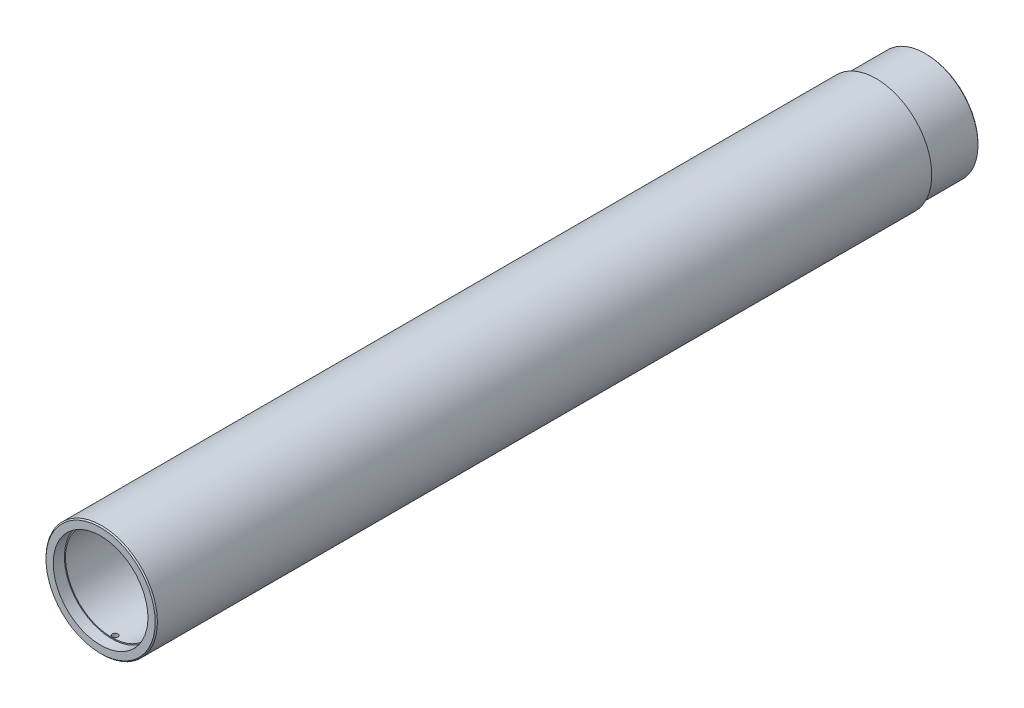
SolidWorks part; units mm, degrees
ref_plane "Front Plane" through (0, 0, 0) normal (0, 0, 1) x (1, 0, 0)
ref_plane "Top Plane" through (0, 0, 0) normal (0, 1, 0) x (1, 0, 0)
ref_plane "Right Plane" through (0, 0, 0) normal (1, 0, 0) x (0, 0, -1)
sketch "Sketch1" plane through (0, 0, 0) normal (0, 0, 1) x (1, 0, 0)
  circle A0 centre (0, 0) radius 50
  circle A1 centre (0, 0) radius 40
  dimension "D1" = 100
  dimension "D2" = 80
extrude "Boss-Extrude1" add sketch "Sketch1" along normal blind 741
sketch "Sketch2" plane through (0, 0, 0) normal (0, 0, -1) x (-1, 0, 0)
  circle A0 centre (0, 0) radius 47.5
  circle A1 centre (0, 0) radius 61.681
  dimension "D1" = 95
extrude "Cut-Extrude1" cut sketch "Sketch2" against normal blind 45
cosmetic thread "Cosmetic Thread1" parameters "D1"=45, "D2"=87.8
chamfer "Chamfer1" distance 1 angle 45 1 edges at (-47.5, 0, 0)
chamfer "Chamfer2" distance 1 angle 45 1 edges at (50, 0, 741)
sketch "Sketch5" plane through (0, 0, 741) normal (0, 0, 1) x (1, 0, 0)
  line L0 (0, 0) -> (-82.1413, 0) construction
  line L1 (-70, 65) -> (70, 65)
  line L2 (-70, 65) -> (-70, 45)
  line L3 (-70, 45) -> (70, 45)
  line L4 (70, 65) -> (70, 45)
  line L5 (-70, -45) -> (70, -45)
  line L6 (-70, -45) -> (-70, -65)
  line L7 (-70, -65) -> (70, -65)
  line L8 (70, -45) -> (70, -65)
  line L9 (0, 0) -> (0, 96.3579) construction
  dimension "D1" = 90
  dimension "D2" = 140
  dimension "D3" = 20
extrude "Cut-Extrude3" [suppressed] cut sketch "Sketch5" against normal blind 15
sketch "Sketch6" plane through (0, 0, 0) normal (1, 0, 0) x (0, 0, -1)
  line L0 (-45, 45) -> (-45, 50)
  line L1 (-45, 50) -> (-40, 50)
  line L2 (-40, 50) -> (-45, 45)
  line L3 (-740, -45) -> (-740, -50)
  line L4 (-740, -50) -> (-735, -50)
  line L5 (-735, -50) -> (-740, -45)
  dimension "D1" = 45
  dimension "D2" = 45
  dimension "D3" = 0
  dimension "D4" = 0
extrude "Cut-Extrude7" [suppressed] cut sketch "Sketch6" against normal through all both and the other way through all
sketch "Sketch7" plane through (0, 0, 45) normal (0, 0, -1) x (-1, 0, 0)
  circle A0 centre (0, 0) radius 42
  dimension "D1" = 84
extrude "Cut-Extrude8" [suppressed] cut sketch "Sketch7" along normal blind 5 flip side to cut
sketch "Sketch10" plane through (0, 0, 741) normal (0, 0, 1) x (1, 0, 0)
  circle A0 centre (0, 0) radius 42.5
  dimension "D1" = 85
extrude "Cut-Extrude9" cut sketch "Sketch10" against normal blind 10
sketch "Sketch11" plane through (0, 0, 731) normal (0, 0, 1) x (1, 0, 0)
  circle A0 centre (0, 0) radius 41.5
  dimension "D1" = 83
extrude "Cut-Extrude10" cut sketch "Sketch11" against normal blind 50
ref_plane "Plane1" through (0, -50, 0) normal (0, 1, 0) x (1, 0, 0)
hole_wizard "M6 Tapped Hole1" positions "Sketch13" profile "Sketch14" tap size "M6" standard "GB"
sketch "Sketch13" plane through (0, -50, 0) normal (0, 1, 0) x (1, 0, 0)
  line L1 (-49, -741) -> (49, -741) construction
  point P4 (0, -728)
  dimension "D1" = 13
sketch "Sketch14" plane through (0, -50, 728) normal (1, 0, 0) x (0, 0, -1)
  line L0 (0, 0) -> (0, 16.5022)
  line L1 (0, 16.5022) -> (2.5, 15)
  line L2 (2.5, 15) -> (2.5, 0)
  line L5 (2.5, 0) -> (0, 0)
  line L10 (0, 16.5022) -> (-2.5, 15) construction
  line L11 (0, -6.35) -> (0, 107.95) construction
  dimension "螺纹孔钻头直径" = 5
  dimension "螺纹孔钻头深度" = 15
  dimension "导头角度" = 118
cosmetic thread "孔螺蚊线1" parameters "D1"=12, "D2"=6
